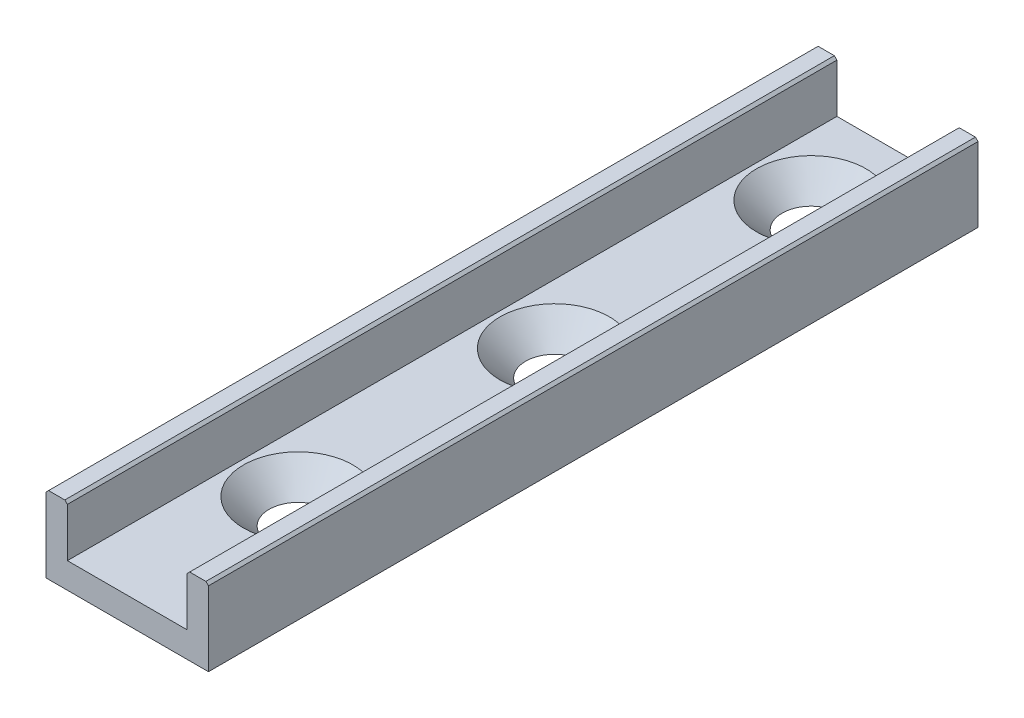
from build123d import *

# Parameters (mm, degrees)
BOSS_EXTRUDE1_DEPTH                         = 90
HOLE_SIZE_PER_HEX_SOCKET_LOBED_SEMI_2_COUNT = 2
HOLE_SIZE_PER_HEX_SOCKET_LOBED_SEMI_2_PITCH = 30
LPATTERN1_COUNT                             = 2
LPATTERN1_PITCH                             = 30
CHAMFER1_SIZE                               = 0.3


with BuildPart() as part:
    # Sketch1 → Boss-Extrude1 (new body)
    with BuildSketch(Plane.XY):
        Polygon((-7, 4.5), (-7, -1.5), (7, -1.5), (7, 4.5), (9.5, 4.5), (9.5, -4.5), (-9.5, -4.5), (-9.5, 4.5), align=None)
    extrude(amount=BOSS_EXTRUDE1_DEPTH)

    # Sketch5 → Hole size per hex socket lobed semi-countersunk screw type1 (revolve, cut)
    with BuildSketch(Plane(origin=(0, -1.5, 10), x_dir=(0, 0, 1), z_dir=(1, 0, 0))):
        Polygon((0, 0), (0, 3), (3.3, 3), (3.3, 3.1), (6.4, 0), align=None)
    hole_size_per_hex_socket_lobed_semi_coun = revolve(axis=Axis((0, 4.85, 10), (0, -1, 0)), mode=Mode.SUBTRACT)

    # Hole size per hex socket lobed semi- 2: Hole size per hex socket lobed semi-countersunk screw type1 ×2
    with Locations(*[(0, 0, i * HOLE_SIZE_PER_HEX_SOCKET_LOBED_SEMI_2_PITCH) for i in range(1, HOLE_SIZE_PER_HEX_SOCKET_LOBED_SEMI_2_COUNT)]):
        add(hole_size_per_hex_socket_lobed_semi_coun, mode=Mode.SUBTRACT)

    # LPattern1: Hole size per hex socket lobed semi-countersunk screw type1 ×2
    with Locations(*[(0, 0, i * LPATTERN1_PITCH) for i in range(1, LPATTERN1_COUNT)]):
        add(hole_size_per_hex_socket_lobed_semi_coun, mode=Mode.SUBTRACT)

    # LPattern1 copy 1 sketch → LPattern1 copy 1 (revolve, cut)
    with BuildSketch(Plane(origin=(0, -1.5, 70), x_dir=(0, 0, 1), z_dir=(1, 0, 0))):
        Polygon((0, 0), (0, 3), (3.3, 3), (3.3, 3.1), (6.4, 0), align=None)
    revolve(axis=Axis((0, 4.85, 70), (0, -1, 0)), mode=Mode.SUBTRACT)

    # Chamfer1
    chamfer1_edges = [part.edges().sort_by_distance(p)[0] for p in [
        (9.5, 4.5, 45),
        (-9.5, 4.5, 45),
        (-7, 4.5, 45),
        (7, 4.5, 45),
    ]]
    chamfer(chamfer1_edges, length=CHAMFER1_SIZE)


solid = part.part
